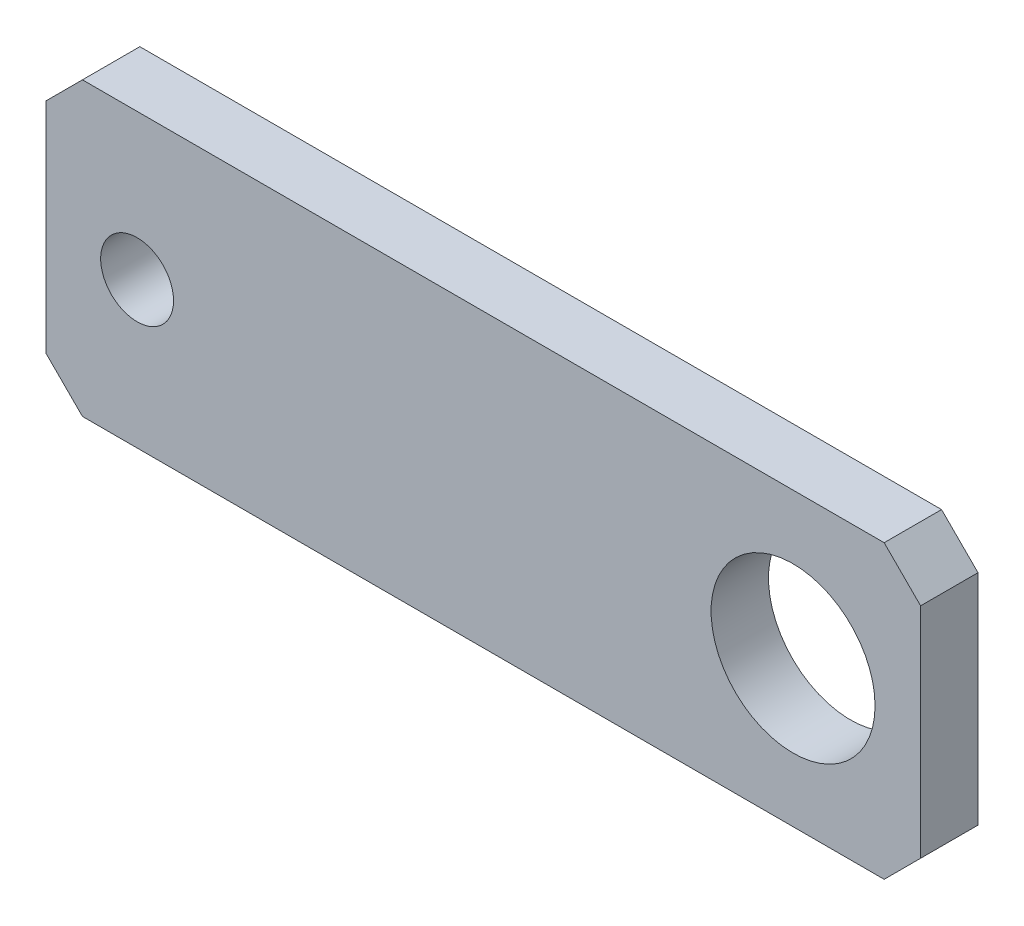
SolidWorks part; units mm, degrees
material "Q235B"
ref_plane "Front Plane" through (0, 0, 0) normal (0, 0, 1) x (1, 0, 0)
ref_plane "Top Plane" through (0, 0, 0) normal (0, 1, 0) x (1, 0, 0)
ref_plane "Right Plane" through (0, 0, 0) normal (1, 0, 0) x (0, 0, -1)
sketch "Sketch1" plane through (0, 0, 0) normal (0, 0, 1) x (1, 0, 0)
  line L0 (0, 0) -> (85.0193, 0) construction
  line L1 (0, 0) -> (0, 54.8732) construction
  line L2 (0, 0) -> (-85.8469, 0) construction
  line L3 (-73.025, 25.4) -> (79.375, 25.4)
  line L4 (-73.025, 25.4) -> (-73.025, -25.4)
  line L5 (-73.025, -25.4) -> (79.375, -25.4)
  line L6 (79.375, 25.4) -> (79.375, -25.4)
  circle A0 centre (57.15, 0) radius 14.2875
  circle A1 centre (-57.15, 0) radius 6.35
  dimension "D3" = 114.3
  dimension "D4" = 28.575
  dimension "D5" = 57.15
  dimension "D6" = 12.7
  dimension "D1" = 50.8
  dimension "D7" = 79.375
  dimension "D8" = 152.4
extrude "Extrude1" add sketch "Sketch1" along normal mid plane 10
chamfer "Chamfer1" distance 6.35 angle 45 4 edges at (-73.025, -25.4, 0) (-73.025, 25.4, 0) (79.375, -25.4, 0) (79.375, 25.4, 0)
